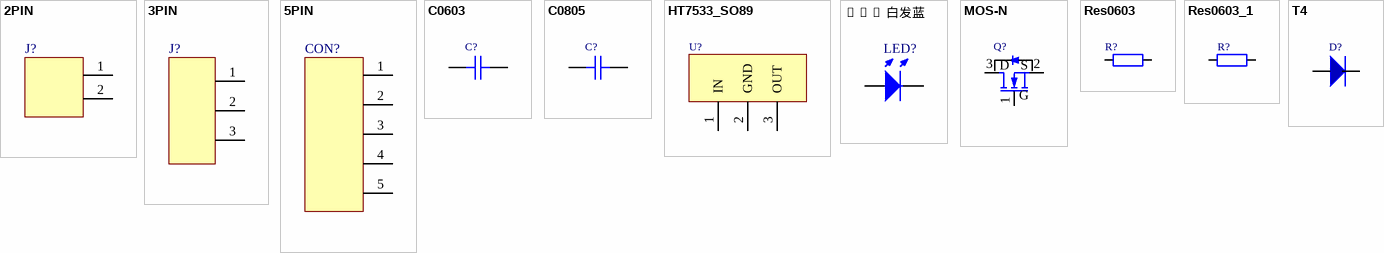
[diagram p0: symbols 2PIN to T4]
# Altium schematic symbol library MISC88840.SCHLIB: 11 symbols
Pins are listed as number, name and electrical type; pins without a type are passive.


## 2PIN
designator J?
DC socket right angle 90°, 2.0 pitch
footprint HY2.0WT-2A/P 立贴带扣耐温260℃ (Horizontal SMD connector)
pins: 1, 2

## 3PIN
designator J?
DC socket 3PIN, 2.0 pitch
footprint 3PIN直插 2.0间距母座 (3PIN through-hole 2.0 pitch female header)
footprint GH1.25-3PIN立贴带扣耐温260℃ (Vertical SMD with latch, heat resistant 260℃)
footprint GH1.25-3PIN立贴带扣耐温260℃ (Vertical SMD with latch, heat resistant 260℃)
pins: 1, 2, 3

## 5PIN
designator CON?
10PIN dual row
footprint 5PIN 2.0间距直插排阵 (5PIN 2.0 pitch through-hole header array)
footprint GH1.25-5PIN立贴带扣耐温260℃ (Vertical SMD with latch, heat resistant 260℃)
pins: 1, 2, 3, 4, 5

## C0603
designator C?
SMD capacitor
footprint C0603 (SMD capacitor C0603)
footprint C0603A (SMD capacitor)
pins: 1, 2

## C0805
designator C?
SMD capacitor
footprint C0805 (SMD capacitor C0805)
footprint C0805A (SMD capacitor)
pins: 1, 2

## HT7533_SO89
designator U?
SMD LDO
footprint TO-252 LDO
footprint TO-252-A
pins: 1 IN, 2 GND, 3 OUT

## LED 白发蓝
designator LED?
SMD LED
footprint 0603-LED-CB
footprint LED-DIP-2
footprint 0603-LED
footprint LED-0603
footprint LED 0603 SMD (LED 0603  SMD)
footprint LED0603A (SMD LED)
pins: 1, 2

## MOS-N
designator Q?
Single N-channel MOSFET
footprint SOT-23-3 MOS
pins: 1 G, 2 S, 3 D

## Res0603
designator R?
SMD resistor
footprint R0603
footprint R0603A (SMD resistor)
pins: 1, 2

## Res0603_1
designator R?
SMD resistor
footprint R0603
footprint R0603A (SMD resistor)
pins: 1, 2

## T4
designator D?
Fast recovery diode
footprint SOD323
pins: 1, 2